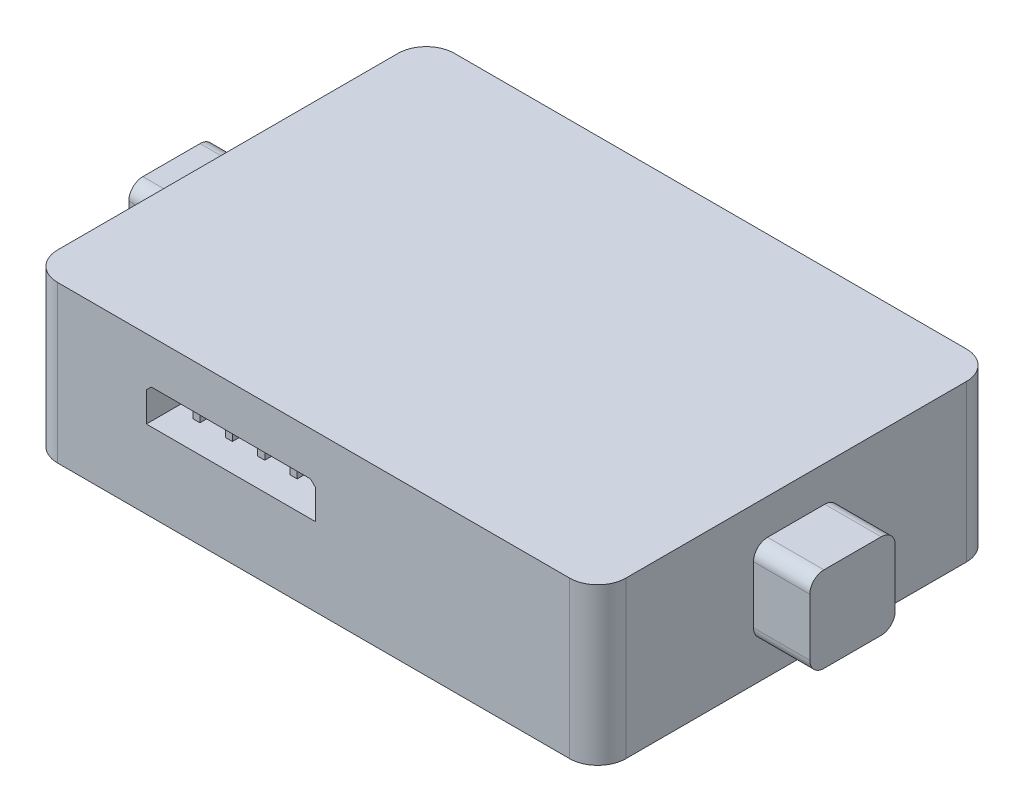
from build123d import *

# Parameters (mm, degrees)
SKETCH_1_W          = 40.33
SKETCH_1_H          = 28.16
EXTRUDE_1_DEPTH     = 11.1
SKETCH_2_W          = 12
SKETCH_2_H          = 2.45
CUT_EXTRUDE_1_DEPTH = 10
SKETCH_3_W          = 0.5
SKETCH_3_H          = 0.5
EXTRUDE_2_DEPTH     = 9
SKETCH_4_W          = 0.5
SKETCH_4_H          = 0.5
EXTRUDE_3_DEPTH     = 9
SKETCH_5_W          = 0.5
SKETCH_5_H          = 0.5
EXTRUDE_4_DEPTH     = 9
SKETCH_6_W          = 0.5
SKETCH_6_H          = 0.5
EXTRUDE_5_DEPTH     = 9
SKETCH_7_W          = 6.06
SKETCH_7_H          = 6.06
EXTRUDE_6_DEPTH     = 4
SKETCH_8_W          = 6.06
SKETCH_8_H          = 6.06
EXTRUDE_7_DEPTH     = 4
CHAMFER_1_SIZE      = 0.35
FILLET_1_R          = 1
FILLET_2_R          = 2


with BuildPart() as part:
    # 草图1 → 凸台-拉伸1 (new body)
    with BuildSketch(Plane(origin=(0, 11.1, 0), x_dir=(1, 0, 0), z_dir=(0, 1, 0))):
        Rectangle(SKETCH_1_W, SKETCH_1_H)
    extrude(amount=-EXTRUDE_1_DEPTH)

    # 草图2 → 切除-拉伸1 (cut)
    with BuildSketch(Plane.XY.offset(14.08)):
        with Locations((-5.865, 6.775)):
            Rectangle(SKETCH_2_W, SKETCH_2_H)
    extrude(amount=-CUT_EXTRUDE_1_DEPTH, mode=Mode.SUBTRACT)

    # 草图3 → 凸台-拉伸2 (add)
    with BuildSketch(Plane.XY.offset(4.08)):
        with Locations((-4.715, 6.775)):
            Rectangle(SKETCH_3_W, SKETCH_3_H)
    extrude(amount=EXTRUDE_2_DEPTH)

    # 草图4 → 凸台-拉伸3 (add)
    with BuildSketch(Plane.XY.offset(4.08)):
        with Locations((-9.315, 6.775)):
            Rectangle(SKETCH_4_W, SKETCH_4_H)
    extrude(amount=EXTRUDE_3_DEPTH)

    # 草图5 → 凸台-拉伸4 (add)
    with BuildSketch(Plane.XY.offset(4.08)):
        with Locations((-7.015, 6.775)):
            Rectangle(SKETCH_5_W, SKETCH_5_H)
    extrude(amount=EXTRUDE_4_DEPTH)

    # 草图6 → 凸台-拉伸5 (add)
    with BuildSketch(Plane.XY.offset(4.08)):
        with Locations((-2.415, 6.775)):
            Rectangle(SKETCH_6_W, SKETCH_6_H)
    extrude(amount=EXTRUDE_5_DEPTH)

    # 草图7 → 凸台-拉伸6 (add)
    with BuildSketch(Plane.ZY.offset(20.165)):
        with Locations((0, 5.55)):
            Rectangle(SKETCH_7_W, SKETCH_7_H)
    extrude(amount=EXTRUDE_6_DEPTH)

    # 草图8 → 凸台-拉伸7 (add)
    with BuildSketch(Plane(origin=(20.165, 0, 0), x_dir=(0, 0, -1), z_dir=(1, 0, 0))):
        with Locations((0, 5.55)):
            Rectangle(SKETCH_8_W, SKETCH_8_H)
    extrude(amount=EXTRUDE_7_DEPTH)

    # 倒角1
    chamfer_1_edges = [part.edges().sort_by_distance(p)[0] for p in [
        (-11.865, 8, 9.08),
        (0.135, 8, 9.08),
    ]]
    chamfer(chamfer_1_edges, length=CHAMFER_1_SIZE)

    # 圆角1
    fillet_1_edges = [part.edges().sort_by_distance(p)[0] for p in [
        (-22.165, 2.52, -3.03),
        (-22.165, 2.52, 3.03),
        (-22.165, 8.58, 3.03),
        (-22.165, 8.58, -3.03),
        (22.165, 2.52, 3.03),
        (22.165, 2.52, -3.03),
        (22.165, 8.58, -3.03),
        (22.165, 8.58, 3.03),
    ]]
    fillet(fillet_1_edges, radius=FILLET_1_R)

    # 圆角2
    fillet_2_edges = [part.edges().sort_by_distance(p)[0] for p in [
        (20.165, 5.55, -14.08),
        (20.165, 5.55, 14.08),
        (-20.165, 5.55, 14.08),
        (-20.165, 5.55, -14.08),
    ]]
    fillet(fillet_2_edges, radius=FILLET_2_R)


solid = part.part
